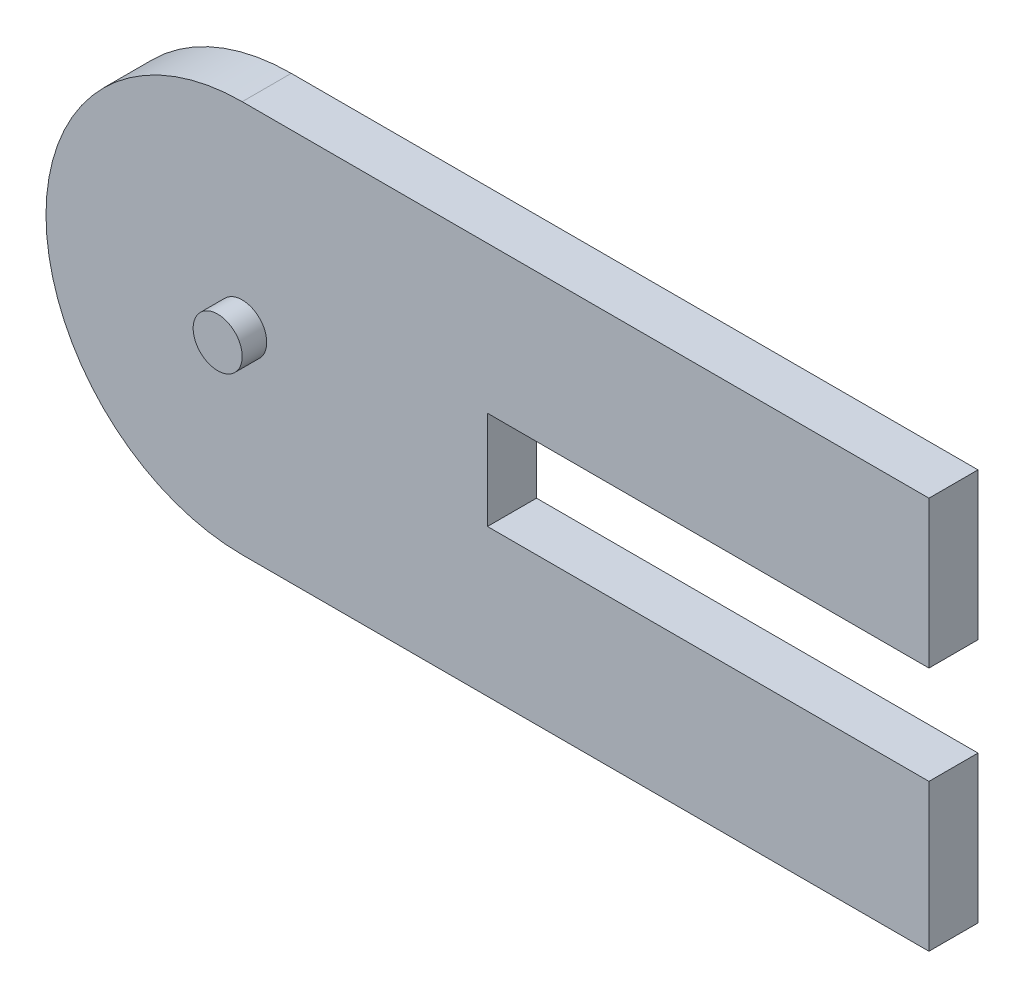
SolidWorks part; units mm, degrees
ref_plane "Plane1" through (0, 0, 0) normal (0, 0, 1) x (1, 0, 0)
ref_plane "Plane2" through (0, 0, 0) normal (0, 1, 0) x (1, 0, 0)
ref_plane "Plane3" through (0, 0, 0) normal (1, 0, 0) x (0, 0, -1)
sketch "Sketch1" plane through (0, 0, 0) normal (0, 0, 1) x (1, 0, 0)
  line L0 (0, 0) -> (140, 0) construction
  line L1 (0, 40) -> (140, 40)
  line L2 (50, 10) -> (140, 10)
  line L3 (140, 40) -> (140, 10)
  line L5 (50, -10) -> (140, -10)
  line L6 (0, -40) -> (140, -40)
  line L7 (140, -40) -> (140, -10)
  line L8 (50, 10) -> (50, -10)
  arc A0 (0, 40) -> (0, -40) centre (0, 0) ccw
  dimension "D1" = 40
  dimension "D2" = 140
  dimension "D3" = 20
  dimension "D4" = 90
extrude "Base-Extrude" add sketch "Sketch1" along normal blind 10
sketch "Sketch2" plane through (0, 0, 10) normal (0, 0, 1) x (1, 0, 0)
  circle A0 centre (0, 0) radius 5
  dimension "D1" = 10
extrude "Boss-Extrude1" add sketch "Sketch2" along normal blind 5
